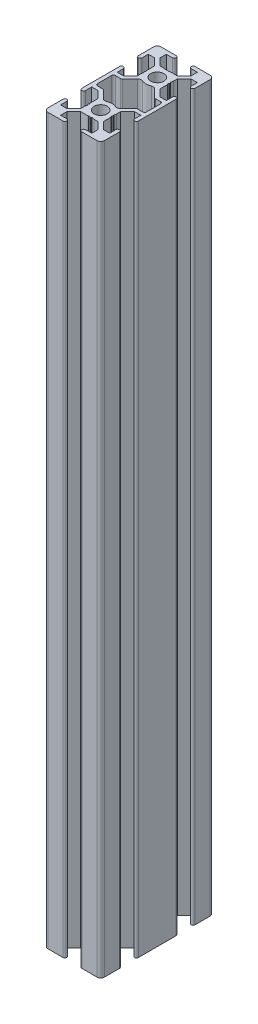
SolidWorks part; units mm, degrees
ref_plane "Front Plane" through (0, 0, 0) normal (0, 0, 1) x (1, 0, 0)
ref_plane "Top Plane" through (0, 0, 0) normal (0, 1, 0) x (1, 0, 0)
ref_plane "Right Plane" through (0, 0, 0) normal (1, 0, 0) x (0, 0, -1)
sketch3d "3DSketch1"
  line L0 (0, 0, 0) -> (0, 384, 0)
  dimension "D1" = 384
other "Aluminium profile 30 X 60 X R2(1)"
ref_plane "Plane1" through (0, 0, 0) normal (0, 1, 0) x (1, 0, 0)
sketch "Sketch11" plane through (0, 0, 0) normal (0, 1, 0) x (1, 0, 0)
  line L0 (-15, -20) -> (-15, -28)
  line L1 (-13, -30) -> (-5, -30)
  line L2 (-5, -28) -> (-8.25, -28)
  line L3 (-8.25, -28) -> (-8.25, -24.6642)
  line L4 (-8.25, -24.6642) -> (-4.5858, -21)
  line L5 (-4.5858, -21) -> (-0.6536, -21)
  line L6 (-0.4036, -20.933) -> (0, -20.7)
  line L7 (0, -20.7) -> (0.4036, -20.933)
  line L8 (0.9036, -20.933) -> (1.2189, -20.751)
  line L9 (1.2189, -20.751) -> (2.5, -21)
  line L10 (2.5, -21) -> (4.5858, -21)
  line L11 (4.5858, -21) -> (8.25, -24.6642)
  line L12 (8.25, -24.6642) -> (8.25, -28)
  line L13 (8.25, -28) -> (5, -28)
  line L14 (5, -30) -> (13, -30)
  line L15 (15, -28) -> (15, -20)
  line L16 (13, -20) -> (13, -23.25)
  line L17 (13, -23.25) -> (9.6642, -23.25)
  line L18 (9.6642, -23.25) -> (6, -19.5858)
  line L19 (6, -19.5858) -> (6, -15.6536)
  line L20 (5.933, -15.4036) -> (5.7, -15)
  line L21 (5.7, -15) -> (5.933, -14.5964)
  line L22 (5.933, -14.0964) -> (5.751, -13.7811)
  line L23 (5.751, -13.7811) -> (6, -12.5)
  line L24 (6, -12.5) -> (6, -10.4142)
  line L25 (6, -10.4142) -> (9.6642, -6.75)
  line L26 (9.6642, -6.75) -> (13, -6.75)
  line L27 (13, -6.75) -> (13, -10)
  line L28 (15, -10) -> (15, 10)
  line L29 (13, 10) -> (13, 6.75)
  line L30 (13, 6.75) -> (9.6642, 6.75)
  line L31 (9.6642, 6.75) -> (6, 10.4142)
  line L32 (6, 10.4142) -> (6, 14.3464)
  line L33 (5.933, 14.5964) -> (5.7, 15)
  line L34 (5.7, 15) -> (5.933, 15.4036)
  line L35 (5.933, 15.9036) -> (5.751, 16.2189)
  line L36 (5.751, 16.2189) -> (6, 17.5)
  line L37 (6, 17.5) -> (6, 19.5858)
  line L38 (6, 19.5858) -> (9.6642, 23.25)
  line L39 (9.6642, 23.25) -> (13, 23.25)
  line L40 (13, 23.25) -> (13, 20)
  line L41 (15, 20) -> (15, 28)
  line L42 (13, 30) -> (5, 30)
  line L43 (5, 28) -> (8.25, 28)
  line L44 (8.25, 28) -> (8.25, 24.6642)
  line L45 (8.25, 24.6642) -> (4.5858, 21)
  line L46 (4.5858, 21) -> (0.6536, 21)
  line L47 (0.4036, 20.933) -> (0, 20.7)
  line L48 (0, 20.7) -> (-0.4036, 20.933)
  line L49 (-0.9036, 20.933) -> (-1.2189, 20.751)
  line L50 (-1.2189, 20.751) -> (-2.5, 21)
  line L51 (-2.5, 21) -> (-4.5858, 21)
  line L52 (-4.5858, 21) -> (-8.25, 24.6642)
  line L53 (-8.25, 24.6642) -> (-8.25, 28)
  line L54 (-8.25, 28) -> (-5, 28)
  line L55 (-5, 30) -> (-13, 30)
  line L56 (-15, 28) -> (-15, 20)
  line L57 (-13, 20) -> (-13, 23.25)
  line L58 (-13, 23.25) -> (-9.6642, 23.25)
  line L59 (-9.6642, 23.25) -> (-6, 19.5858)
  line L60 (-6, 19.5858) -> (-6, 15.6536)
  line L61 (-5.933, 15.4036) -> (-5.7, 15)
  line L62 (-5.7, 15) -> (-5.933, 14.5964)
  line L63 (-5.933, 14.0964) -> (-5.751, 13.7811)
  line L64 (-5.751, 13.7811) -> (-6, 12.5)
  line L65 (-6, 12.5) -> (-6, 10.4142)
  line L66 (-6, 10.4142) -> (-9.6642, 6.75)
  line L67 (-9.6642, 6.75) -> (-13, 6.75)
  line L68 (-13, 6.75) -> (-13, 10)
  line L69 (-15, 10) -> (-15, -10)
  line L70 (-13, -10) -> (-13, -6.75)
  line L71 (-13, -6.75) -> (-9.6642, -6.75)
  line L72 (-9.6642, -6.75) -> (-6, -10.4142)
  line L73 (-6, -10.4142) -> (-6, -14.3464)
  line L74 (-5.933, -14.5964) -> (-5.7, -15)
  line L75 (-5.7, -15) -> (-5.933, -15.4036)
  line L76 (-5.933, -15.9036) -> (-5.751, -16.2189)
  line L77 (-5.751, -16.2189) -> (-6, -17.5)
  line L78 (-6, -17.5) -> (-6, -19.5858)
  line L79 (-6, -19.5858) -> (-9.6642, -23.25)
  line L80 (-9.6642, -23.25) -> (-13, -23.25)
  line L81 (-13, -23.25) -> (-13, -20)
  line L82 (-13, 3.75) -> (-13, -3.75)
  line L83 (-12, -4.75) -> (-9.25, -4.75)
  line L84 (-8.5429, -5.0429) -> (-4.5369, -9.0488)
  line L85 (4.5369, -9.0488) -> (8.5429, -5.0429)
  line L86 (9.25, -4.75) -> (12, -4.75)
  line L87 (13, -3.75) -> (13, 3.75)
  line L88 (12, 4.75) -> (9.25, 4.75)
  line L89 (8.5429, 5.0429) -> (4.5369, 9.0488)
  line L90 (-4.5369, 9.0488) -> (-8.5429, 5.0429)
  line L91 (-9.25, 4.75) -> (-12, 4.75)
  arc A0 (-15, -28) -> (-13, -30) centre (-13, -28) ccw
  arc A1 (-5, -30) -> (-5, -28) centre (-5, -29) ccw
  arc A2 (-0.6536, -21) -> (-0.4036, -20.933) centre (-0.6536, -20.5) ccw
  arc A3 (0.4036, -20.933) -> (0.9036, -20.933) centre (0.6536, -20.5) ccw
  arc A4 (5, -28) -> (5, -30) centre (5, -29) ccw
  arc A5 (13, -30) -> (15, -28) centre (13, -28) ccw
  arc A6 (15, -20) -> (13, -20) centre (14, -20) ccw
  arc A7 (6, -15.6536) -> (5.933, -15.4036) centre (5.5, -15.6536) ccw
  arc A8 (5.933, -14.5964) -> (5.933, -14.0964) centre (5.5, -14.3464) ccw
  arc A9 (13, -10) -> (15, -10) centre (14, -10) ccw
  arc A10 (15, 10) -> (13, 10) centre (14, 10) ccw
  arc A11 (6, 14.3464) -> (5.933, 14.5964) centre (5.5, 14.3464) ccw
  arc A12 (5.933, 15.4036) -> (5.933, 15.9036) centre (5.5, 15.6536) ccw
  arc A13 (13, 20) -> (15, 20) centre (14, 20) ccw
  arc A14 (15, 28) -> (13, 30) centre (13, 28) ccw
  arc A15 (5, 30) -> (5, 28) centre (5, 29) ccw
  arc A16 (0.6536, 21) -> (0.4036, 20.933) centre (0.6536, 20.5) ccw
  arc A17 (-0.4036, 20.933) -> (-0.9036, 20.933) centre (-0.6536, 20.5) ccw
  arc A18 (-5, 28) -> (-5, 30) centre (-5, 29) ccw
  arc A19 (-13, 30) -> (-15, 28) centre (-13, 28) ccw
  arc A20 (-15, 20) -> (-13, 20) centre (-14, 20) ccw
  arc A21 (-6, 15.6536) -> (-5.933, 15.4036) centre (-5.5, 15.6536) ccw
  arc A22 (-5.933, 14.5964) -> (-5.933, 14.0964) centre (-5.5, 14.3464) ccw
  arc A23 (-13, 10) -> (-15, 10) centre (-14, 10) ccw
  arc A24 (-15, -10) -> (-13, -10) centre (-14, -10) ccw
  arc A25 (-6, -14.3464) -> (-5.933, -14.5964) centre (-5.5, -14.3464) ccw
  arc A26 (-5.933, -15.4036) -> (-5.933, -15.9036) centre (-5.5, -15.6536) ccw
  arc A27 (-13, -20) -> (-15, -20) centre (-14, -20) ccw
  arc A28 (-13, -3.75) -> (-12, -4.75) centre (-12, -3.75) ccw
  arc A29 (-9.25, -4.75) -> (-8.5429, -5.0429) centre (-9.25, -5.75) cw
  arc A30 (-4.5369, -9.0488) -> (-2.342, -9.476) centre (-3.1227, -7.6346) ccw
  arc A31 (-2.342, -9.476) -> (2.342, -9.476) centre (0, -15) cw
  arc A32 (2.342, -9.476) -> (4.5369, -9.0488) centre (3.1227, -7.6346) ccw
  arc A33 (8.5429, -5.0429) -> (9.25, -4.75) centre (9.25, -5.75) cw
  arc A34 (12, -4.75) -> (13, -3.75) centre (12, -3.75) ccw
  arc A35 (13, 3.75) -> (12, 4.75) centre (12, 3.75) ccw
  arc A36 (9.25, 4.75) -> (8.5429, 5.0429) centre (9.25, 5.75) cw
  arc A37 (4.5369, 9.0488) -> (2.342, 9.476) centre (3.1227, 7.6346) ccw
  arc A38 (2.342, 9.476) -> (-2.342, 9.476) centre (0, 15) cw
  arc A39 (-2.342, 9.476) -> (-4.5369, 9.0488) centre (-3.1227, 7.6346) ccw
  arc A40 (-8.5429, 5.0429) -> (-9.25, 4.75) centre (-9.25, 5.75) cw
  arc A41 (-12, 4.75) -> (-13, 3.75) centre (-12, 3.75) ccw
  circle A42 centre (0, 15) radius 3.4
  circle A43 centre (0, -15) radius 3.4
  point P178 (0, 0)
  point P179 (0, 0)
  dimension "D3" = 6.8
  dimension "D1" = 30
  dimension "D2" = 60
hole_wizard "M8x1.0 Tapped Hole1" positions "Sketch14" profile "Sketch15" tap size "M8x1.0" standard "GB"
sketch "Sketch14" plane through (0, 384, 0) normal (0, 1, 0) x (1, 0, 0)
  point P0 (0, 15)
  point P4 (0, -15)
cosmetic thread "Hole thread line1"
cosmetic thread "Hole thread line2"
sketch "Sketch15" plane through (0, 384, -15) normal (1, 0, 0) x (0, 0, 1)
  line L0 (0, 0) -> (0, 391.103)
  line L1 (0, 391.103) -> (3.5, 389)
  line L2 (3.5, 389) -> (3.5, 0)
  line L5 (3.5, 0) -> (0, 0)
  line L10 (0, 391.103) -> (-3.5, 389) construction
  line L11 (0, -6.35) -> (0, 107.95) construction
  dimension "螺纹孔钻头直径" = 7
  dimension "螺纹孔钻头深度" = 389
  dimension "导头角度" = 118
hole_wizard "M8x1.0 Tapped Hole2" positions "3DSketch2" profile "Sketch17" tap size "M8x1.0" standard "GB"
sketch3d "3DSketch2"
  line L0 (0, 0, -15) -> (0, 384, -15) construction
  line L1 (0, 0, 15) -> (0, 384, 15) construction
  point P0 (0, 0, -15)
  point P5 (0, 0, 15)
sketch "Sketch17" plane through (0, 0, -15) normal (1, 0, 0) x (0, 0, -1)
  line L0 (0, 0) -> (0, 17.103)
  line L1 (0, 17.103) -> (3.5, 15)
  line L2 (3.5, 15) -> (3.5, 0)
  line L5 (3.5, 0) -> (0, 0)
  line L10 (0, 17.103) -> (-3.5, 15) construction
  line L11 (0, -6.35) -> (0, 107.95) construction
  dimension "螺纹孔钻头直径" = 7
  dimension "螺纹孔钻头深度" = 15
  dimension "导头角度" = 118
cosmetic thread "Hole thread line3"
cosmetic thread "Hole thread line4"
equation "\"1\"= \"代号代号\""
equation "\"2\"= \"名称代号\""
